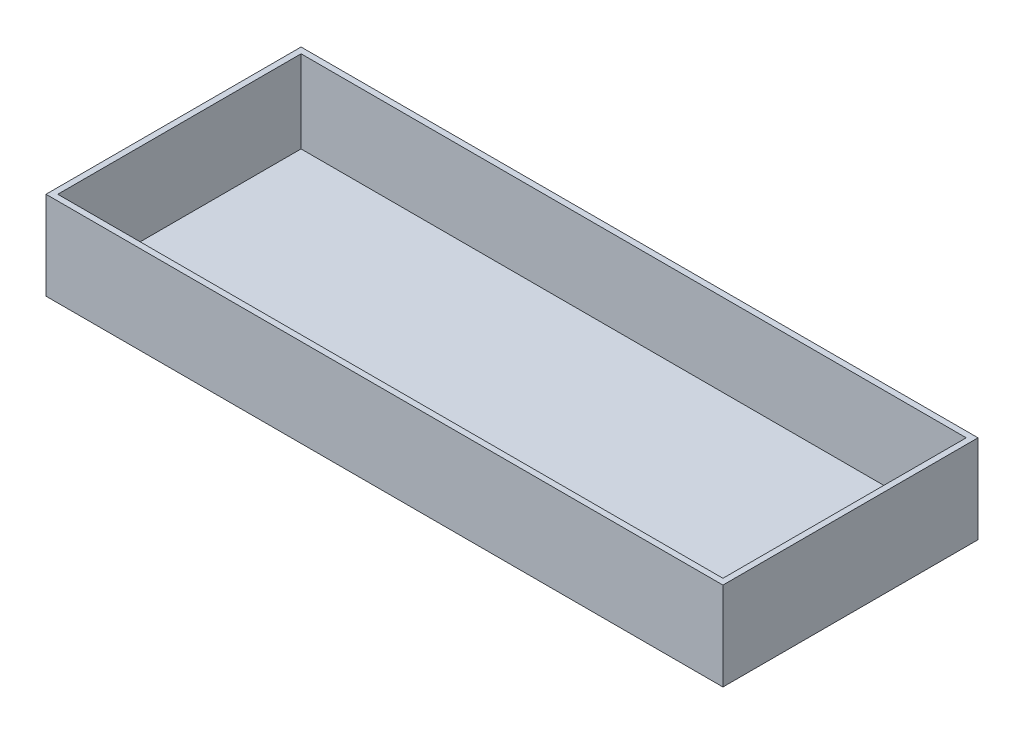
from build123d import *

# Parameters (mm, degrees)
SKETCH1_W           = 690
SKETCH1_H           = 260
BOSS_EXTRUDE1_DEPTH = 90
SHELL1_T            = -6


with BuildPart() as part:
    # Sketch1 → Boss-Extrude1 (new body)
    with BuildSketch(Plane(origin=(0, 0, 0), x_dir=(1, 0, 0), z_dir=(0, 1, 0))):
        Rectangle(SKETCH1_W, SKETCH1_H)
    extrude(amount=BOSS_EXTRUDE1_DEPTH)

    # Shell1
    shell1_openings = [part.faces().sort_by_distance(p)[0] for p in [
        (0, 90, 0),
    ]]
    offset(amount=SHELL1_T, openings=shell1_openings, kind=Kind.INTERSECTION)


solid = part.part
